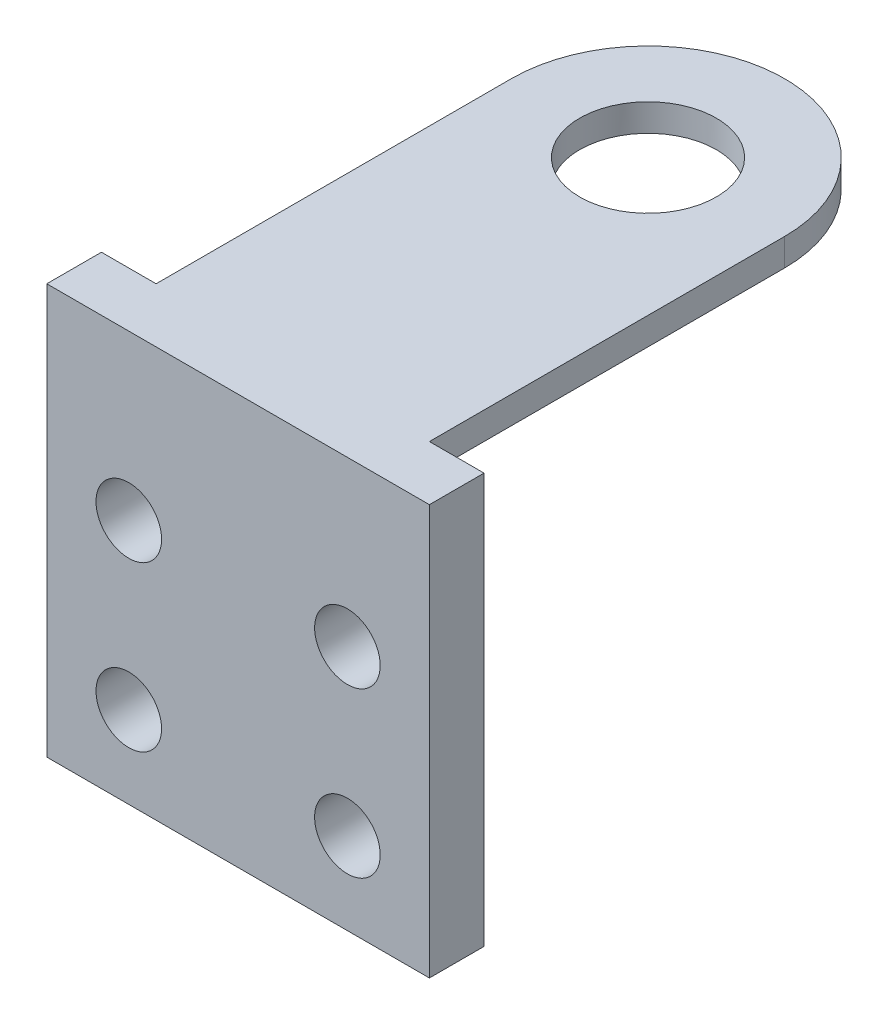
from build123d import *

# Parameters (mm, degrees)
SKETCH_1_W          = 70
SKETCH_1_H          = 70
SKETCH_1_R          = 6
EXTRUDE_1_DEPTH     = 10
SKETCH_2_W          = 70
SKETCH_2_H          = 5
EXTRUDE_2_DEPTH     = 100
SKETCH_4_R          = 12.5
CUT_EXTRUDE_1_DEPTH = 10


with BuildPart() as part:
    # 草图1 → 凸台-拉伸1 (new body)
    with BuildSketch(Plane.XY):
        with Locations((20, 20)):
            Rectangle(SKETCH_1_W, SKETCH_1_H)
        Circle(SKETCH_1_R, mode=Mode.SUBTRACT)
        with Locations((0, 30)):
            Circle(SKETCH_1_R, mode=Mode.SUBTRACT)
        with Locations((40, 30)):
            Circle(SKETCH_1_R, mode=Mode.SUBTRACT)
        with Locations((40, 0)):
            Circle(SKETCH_1_R, mode=Mode.SUBTRACT)
    extrude(amount=EXTRUDE_1_DEPTH)

    # 草图2 → 凸台-拉伸2 (add)
    with BuildSketch(Plane.XY.offset(10)):
        with Locations((20, 57.5)):
            Rectangle(SKETCH_2_W, SKETCH_2_H)
    extrude(amount=-EXTRUDE_2_DEPTH)

    # 草图4 → 切除-拉伸1 (cut)
    with BuildSketch(Plane(origin=(0, 60, 0), x_dir=(1, 0, 0), z_dir=(0, 1, 0))):
        with Locations(Location((20, 65, 0), (0, 0, 270))):
            Circle(SKETCH_4_R)
        with BuildLine():
            Line((-5, 65), (-5, 0))
            Line((-5, 0), (-73.267990544, 0))
            Line((-73.267990544, 0), (-73.267990544, 50))
            Line((-73.267990544, 50), (-73.267990544, 103.705684911))
            Line((-73.267990544, 103.705684911), (78.593427938, 103.705684911))
            Line((78.593427938, 103.705684911), (78.593427938, 0))
            Line((78.593427938, 0), (45, 0))
            Line((45, 0), (45, 65))
            ThreePointArc((45, 65), (20, 90), (-5, 65))
        make_face()
    extrude(amount=-CUT_EXTRUDE_1_DEPTH, mode=Mode.SUBTRACT)


solid = part.part
